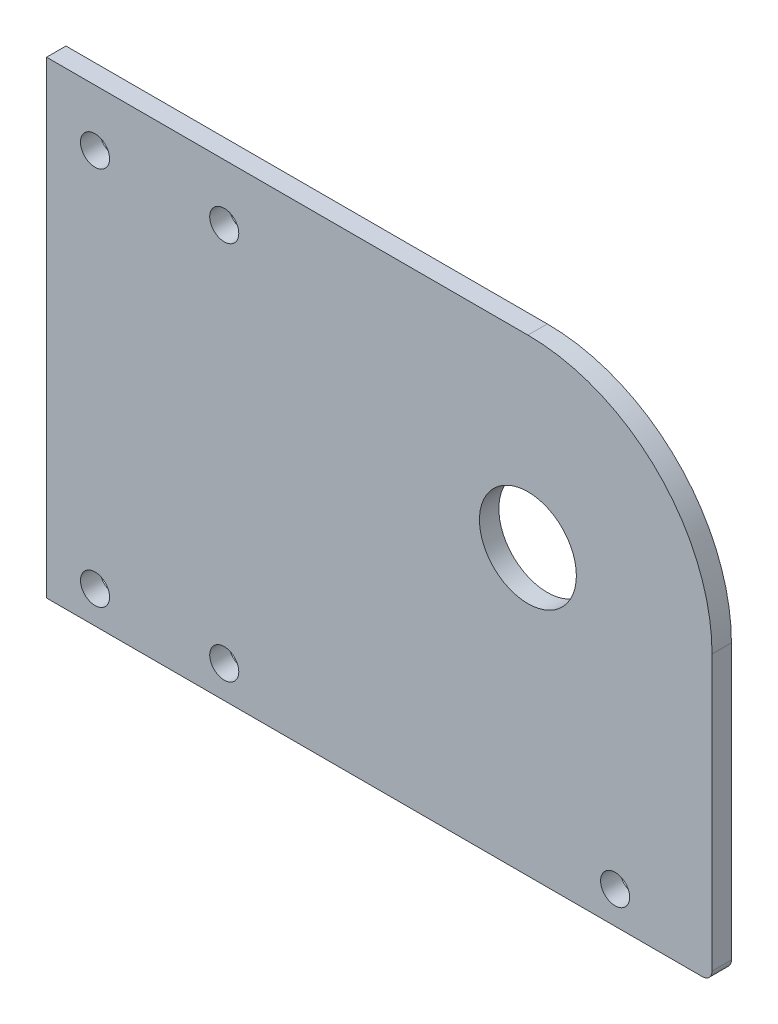
SolidWorks part; units mm, degrees
material "普通碳钢"
ref_plane "前视基准面" through (0, 0, 0) normal (0, 0, 1) x (1, 0, 0)
ref_plane "上视基准面" through (0, 0, 0) normal (0, 1, 0) x (1, 0, 0)
ref_plane "右视基准面" through (0, 0, 0) normal (1, 0, 0) x (0, 0, -1)
sketch "草图1" plane through (0, 0, 0) normal (0, 0, 1) x (1, 0, 0)
  line L0 (0, 72.5) -> (0, 0) construction
  line L1 (-103, 72.5) -> (103, 72.5)
  line L2 (-103, 72.5) -> (-103, -72.5)
  line L3 (-103, -72.5) -> (103, -72.5)
  line L4 (103, 72.5) -> (103, -72.5)
  line L5 (0, 0) -> (103, 0) construction
  dimension "D1" = 206
  dimension "D2" = 145
extrude "凸台-拉伸1" add sketch "草图1" along normal blind 6
sketch "草图2" plane through (0, 0, 6) normal (0, 0, 1) x (1, 0, 0)
  line L0 (103, 72.5) -> (-103, 72.5) construction
  line L1 (-103, -72.5) -> (-3, -72.5)
  line L2 (-103, -72.5) -> (-103, -7.5)
  line L3 (-103, -7.5) -> (-3, -7.5)
  line L4 (-3, -72.5) -> (-3, -7.5)
  dimension "D1" = 80
  dimension "D2" = 100
extrude "切除-拉伸1" [suppressed] cut sketch "草图2" against normal through all
sketch "草图3" plane through (0, 0, 6) normal (0, 0, 1) x (1, 0, 0)
  line L0 (103, 72.5) -> (-103, 72.5) construction
  line L1 (-103, 72.5) -> (-103, -72.5) construction
  circle A0 centre (-88, 55) radius 4.5
  circle A1 centre (-48, 55) radius 4.5
  circle A2 centre (-88, -62.5) radius 4.5
  circle A3 centre (-48, -62.5) radius 4.5
  dimension "D1" = 9
  dimension "D2" = 40
  dimension "D3" = 117.5
  dimension "D4" = 17.5
  dimension "D5" = 15
extrude "切除-拉伸2" cut sketch "草图3" against normal through all
sketch "草图4" plane through (0, 0, 6) normal (0, 0, 1) x (1, 0, 0)
  line L0 (103, 72.5) -> (-103, 72.5) construction
  line L2 (103, -72.5) -> (103, 72.5) construction
  circle A0 centre (46, 15.5) radius 15
  dimension "D1" = 30
  dimension "D3" = 57
  dimension "D2" = 57
extrude "切除-拉伸3" cut sketch "草图4" against normal through all
fillet "圆角1" radius 57 1 edges at (103, 72.5, 3)
fillet "圆角2" [suppressed] radius 10
fillet "圆角3" [suppressed] radius 10
sketch "草图5" plane through (0, 0, 6) normal (0, 0, 1) x (1, 0, 0)
  line L0 (46, 72.5) -> (-103, 72.5) construction
  line L1 (103, -72.5) -> (103, 15.5) construction
  circle A0 centre (88, 61) radius 2.75
  dimension "D1" = 11.5
  dimension "D2" = 5.5
  dimension "D3" = 15
extrude "切除-拉伸4" [suppressed] cut sketch "草图5" against normal through all
hole_wizard "M10 螺纹孔1" positions "草图7" profile "草图6" tap size "M10" standard "Gb"
sketch "草图7" plane through (0, 0, 8) normal (0, 0, 1) x (1, 0, 0)
  line L0 (44, 41.9926) -> (44, 5) construction
  line L1 (44, 5) -> (88.8291, 5) construction
  point P0 (5.75, 5)
  dimension "D1" = 38.25
cosmetic thread "孔螺蚊线1" [suppressed] parameters "D2"=10
sketch "草图6" plane through (5.75, 5, 8) normal (1, 0, 0) x (0, -1, 0)
  line L0 (0, 0) -> (0, 8)
  line L1 (0, 8) -> (4.25, 8)
  line L2 (4.25, 8) -> (4.25, 0)
  line L5 (4.25, 0) -> (0, 0)
  line L11 (0, -6.35) -> (0, 107.95) construction
  dimension "通孔螺纹孔钻头直径" = 8.5
  dimension "通孔螺纹孔钻头深度" = 8
pattern_circular "阵列(圆周)1" [suppressed] count 2 over 360
sketch "草图8" plane through (0, 0, 6) normal (0, 0, 1) x (1, 0, 0)
  line L1 (103, -72.5) -> (98, -72.5)
  line L2 (103, -72.5) -> (103, -27.5)
  line L3 (103, -27.5) -> (98, -27.5)
  line L4 (98, -72.5) -> (98, -27.5)
  dimension "D1" = 5
  dimension "D2" = 45
extrude "切除-拉伸5" [suppressed] cut sketch "草图8" against normal through all
hole_wizard "M4 螺纹孔1" positions "草图10" profile "草图9" tap size "M4" standard "Iso"
sketch "草图10" [suppressed] plane through (98, 0, 0) normal (1, 0, 0) x (0, 0, -1)
  line L0 (-4, -72.5) -> (-4, -20.2113) construction
  line L1 (0, -72.5) -> (-8, -72.5) construction
  point P0 (-4, -62.5)
  point P2 (-4, -37.5)
  dimension "D1" = 10
  dimension "D2" = 25
sketch "草图9" plane through (98, -62.5, 4) normal (0, 1, 0) x (0, 0, -1)
  line L0 (0, 0) -> (0, 12.4914)
  line L1 (0, 12.4914) -> (1.65, 11.5)
  line L2 (1.65, 11.5) -> (1.65, 0)
  line L5 (1.65, 0) -> (0, 0)
  line L10 (0, 12.4914) -> (-1.65, 11.5) construction
  line L11 (0, -6.35) -> (0, 107.95) construction
  dimension "螺纹孔钻头直径" = 3.3
  dimension "螺纹孔钻头深度" = 11.5
  dimension "导头角度" = 118
cosmetic thread "孔螺蚊线2" [suppressed] parameters "D1"=8, "D2"=4
cosmetic thread "孔螺蚊线3" [suppressed] parameters "D1"=8, "D2"=4
fillet "圆角4" [suppressed] radius 3
sketch "草图11" plane through (0, 0, 6) normal (0, 0, 1) x (1, 0, 0)
  line L1 (-103, -72.5) -> (103, -72.5) construction
  line L2 (103, -72.5) -> (103, 15.5) construction
  circle A0 centre (73, -62.5) radius 4.5
  dimension "D1" = 9
  dimension "D2" = 10
  dimension "D3" = 30
extrude "切除-拉伸6" cut sketch "草图11" against normal through all
fillet "圆角5" radius 3 1 edges at (103, -72.5, 3)
